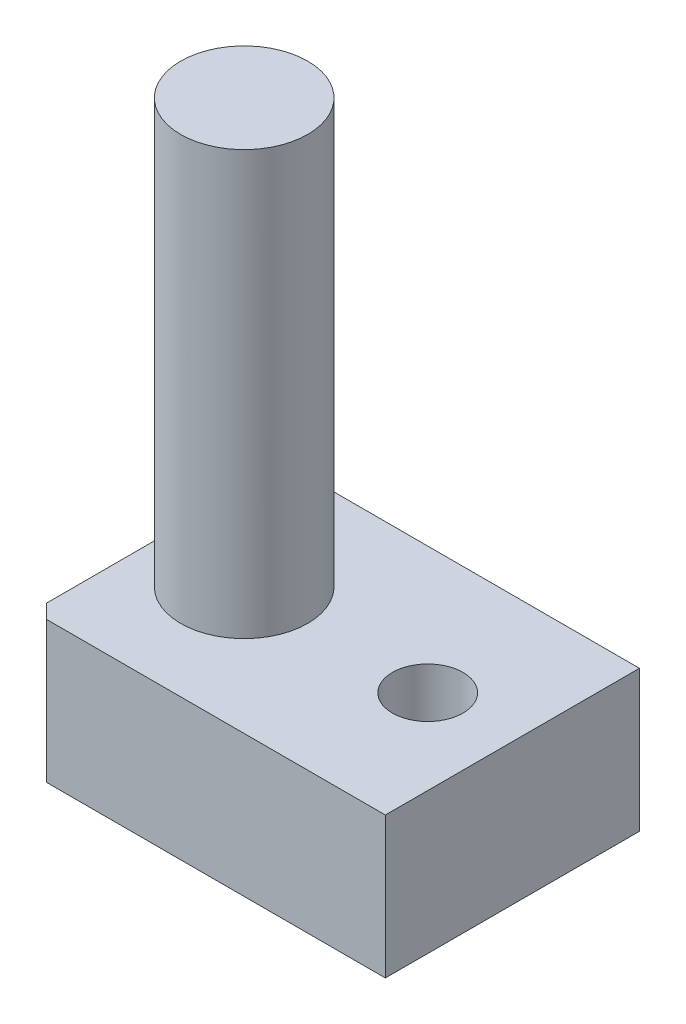
SolidWorks part; units mm, degrees
ref_plane "前视基准面" through (0, 0, 0) normal (0, 0, 1) x (1, 0, 0)
ref_plane "上视基准面" through (0, 0, 0) normal (0, 1, 0) x (1, 0, 0)
ref_plane "右视基准面" through (0, 0, 0) normal (1, 0, 0) x (0, 0, -1)
sketch "草图1" plane through (0, 0, 0) normal (0, 0, 1) x (1, 0, 0)
  line L1 (12.5, -5) -> (-12.5, -5)
  line L2 (12.5, -5) -> (12.5, 5)
  line L3 (12.5, 5) -> (-12.5, 5)
  line L4 (-12.5, -5) -> (-12.5, 5)
  line L5 (12.5, -5) -> (-12.5, 5) construction
  line L6 (12.5, 5) -> (-12.5, -5) construction
  point P0 (0, 0)
  dimension "D1" = 10
  dimension "D2" = 25
extrude "凸台-拉伸1" add sketch "草图1" along normal blind 18
sketch "草图2" plane through (0, 5, 0) normal (0, 1, 0) x (1, 0, 0)
  line L0 (-12.5, -9) -> (-6.5, -9) construction
  line L1 (-12.5, -18) -> (-12.5, 0) construction
  circle A0 centre (-6.5, -9) radius 4.5
  dimension "D2" = 9
  dimension "D1" = 6
extrude "凸台-拉伸2" add sketch "草图2" along normal blind 30
sketch "草图3" plane through (0, 5, 0) normal (0, 1, 0) x (1, 0, 0)
  line L0 (6.5, -9) -> (12.5, -9) construction
  line L1 (12.5, -18) -> (12.5, 0) construction
  circle A0 centre (6.5, -9) radius 2.5
  dimension "D2" = 5
  dimension "D1" = 6
extrude "切除-拉伸1" cut sketch "草图3" against normal up to next
chamfer "倒角1" distance 1 angle 45 2 edges at (-12.5, 0, 18) (-12.5, 0, 0)
